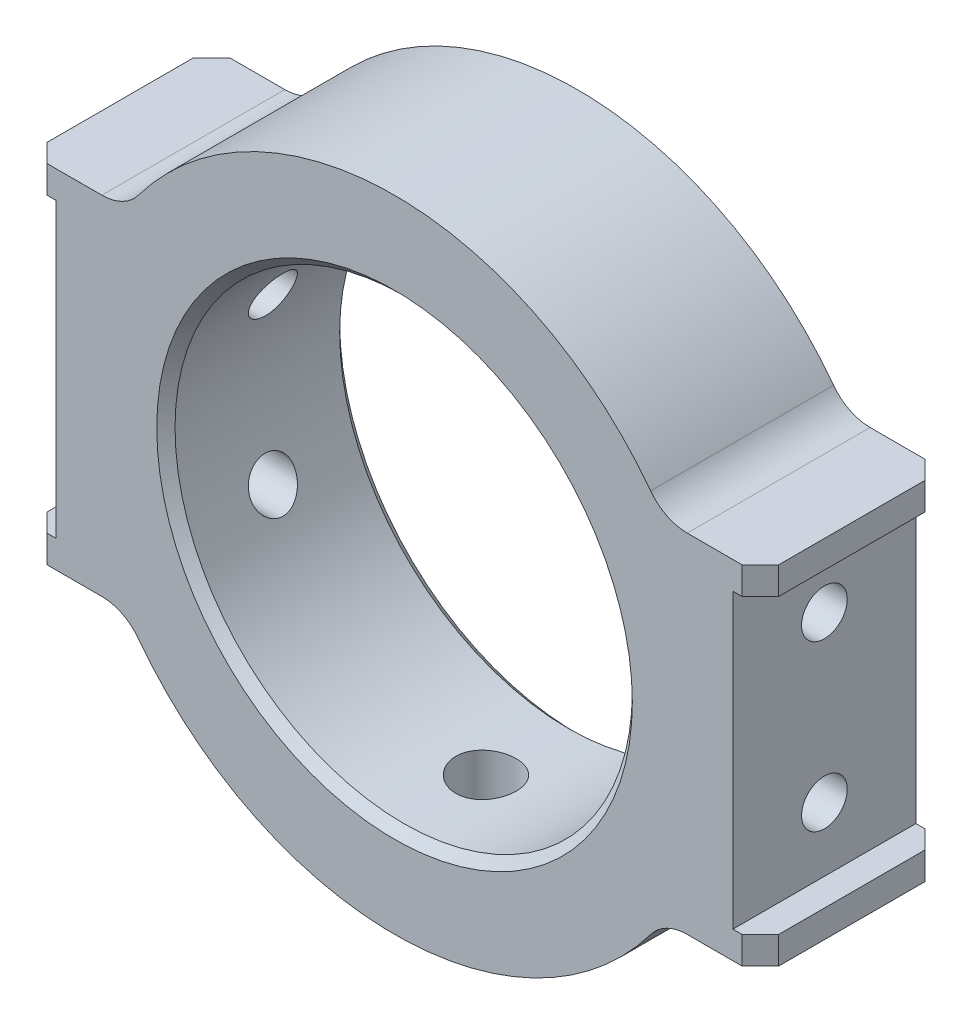
SolidWorks part; units mm, degrees
ref_plane "Front Plane" through (0, 0, 0) normal (0, 0, 1) x (1, 0, 0)
ref_plane "Top Plane" through (0, 0, 0) normal (0, 1, 0) x (1, 0, 0)
ref_plane "Right Plane" through (0, 0, 0) normal (1, 0, 0) x (0, 0, -1)
sketch "Sketch1" plane through (0, 0, 0) normal (0, 0, 1) x (1, 0, 0)
  circle A0 centre (0, 0) radius 17.5
  dimension "D1" = 35
extrude "Boss-Extrude1" add sketch "Sketch1" along normal blind 10
sketch "Sketch2" plane through (0, 0, 10) normal (0, 0, 1) x (1, 0, 0)
  line L1 (-20, -9.5) -> (20, -9.5)
  line L2 (-20, -9.5) -> (-20, 9.5)
  line L3 (-20, 9.5) -> (20, 9.5)
  line L4 (20, -9.5) -> (20, 9.5)
  line L5 (-20, -9.5) -> (20, 9.5) construction
  line L6 (-20, 9.5) -> (20, -9.5) construction
  point P0 (0, 0)
  dimension "D1" = 19
  dimension "D2" = 40
extrude "Boss-Extrude2" add sketch "Sketch2" against normal up to surface (10 mm away) up to face at (17.5, 0, 0)
chamfer "Chamfer1" distance 1 angle 45 4 edges at (20, 0, 0) (20, 0, 10) (-20, 0, 0) (-20, 0, 10)
sketch "Sketch3" plane through (0, 0, 10) normal (0, 0, 1) x (1, 0, 0)
  circle A0 centre (0, 0) radius 12.5
  dimension "D1" = 25
extrude "Cut-Extrude1" cut sketch "Sketch3" against normal through all
sketch "Sketch4" plane through (0, 0, 10) normal (0, 0, 1) x (1, 0, 0)
  line L0 (20, -9.5) -> (20, 9.5) construction
  line L1 (21.5, -8) -> (18.5, -8)
  line L2 (21.5, -8) -> (21.5, 8)
  line L3 (21.5, 8) -> (18.5, 8)
  line L4 (18.5, -8) -> (18.5, 8)
  line L5 (21.5, -8) -> (18.5, 8) construction
  line L6 (21.5, 8) -> (18.5, -8) construction
  line L7 (-20, 9.5) -> (-20, -9.5) construction
  line L8 (-21.5, -8) -> (-18.5, -8)
  line L9 (-21.5, -8) -> (-21.5, 8)
  line L10 (-21.5, 8) -> (-18.5, 8)
  line L11 (-18.5, -8) -> (-18.5, 8)
  line L12 (-21.5, -8) -> (-18.5, 8) construction
  line L13 (-21.5, 8) -> (-18.5, -8) construction
  point P0 (20, 0)
  point P7 (-20, 0)
  dimension "D1" = 16
  dimension "D2" = 1.5
extrude "Cut-Extrude2" cut sketch "Sketch4" against normal through all
ref_plane "Plane1" through (0, -20.3528, 0) normal (0, 1, 0) x (1, 0, 0)
hole_wizard "M4 Tapped Hole1" positions "Sketch6" profile "Sketch5" tap size "M4" standard "Gb"
sketch "Sketch6" plane through (0, -20.3528, 0) normal (0, 1, 0) x (1, 0, 0)
  line L0 (0, -10) -> (0, 0) construction
  line L1 (-14.6969, -10) -> (14.6969, -10) construction
  point P0 (0, -5)
sketch "Sketch5" plane through (0, -20.3528, 5) normal (1, 0, 0) x (0, 0, -1)
  line L0 (0, 0) -> (0, 11.0914)
  line L1 (0, 11.0914) -> (1.65, 10.1)
  line L2 (1.65, 10.1) -> (1.65, 0)
  line L5 (1.65, 0) -> (0, 0)
  line L10 (0, 11.0914) -> (-1.65, 10.1) construction
  line L11 (0, -6.35) -> (0, 107.95) construction
  dimension "螺纹孔钻头直径" = 3.3
  dimension "螺纹孔钻头深度" = 10.1
  dimension "导头角度" = 118
cosmetic thread "Hole thread 1" parameters "D1"=7.9622, "D2"=4
fillet "Fillet1" radius 2.5 4 edges at (14.6969, 9.5, 5) (-14.6969, 9.5, 5) (-14.6969, -9.5, 5) (14.6969, -9.5, 5)
hole_wizard "M3 Tapped Hole1" positions "Sketch8" profile "Sketch7" tap size "M3" standard "Gb"
sketch "Sketch8" plane through (18.5, 0, 0) normal (1, 0, 0) x (0, 0, -1)
  line L0 (-5, -8) -> (-5, 8) construction
  line L1 (0, -8) -> (-10, -8) construction
  line L2 (-1, 8) -> (-9, 8) construction
  line L4 (-5, 0) -> (-13.3246, 0) construction
  point P0 (-5, -4.5)
  point P2 (-5, 4.5)
  dimension "D1" = 9
sketch "Sketch7" plane through (18.5, -4.5, 5) normal (0, 1, 0) x (0, 0, -1)
  line L0 (0, 0) -> (0, 8.2511)
  line L1 (0, 8.2511) -> (1.25, 7.5)
  line L2 (1.25, 7.5) -> (1.25, 0)
  line L5 (1.25, 0) -> (0, 0)
  line L10 (0, 8.2511) -> (-1.25, 7.5) construction
  line L11 (0, -6.35) -> (0, 107.95) construction
  dimension "螺纹孔钻头直径" = 2.5
  dimension "螺纹孔钻头深度" = 7.5
  dimension "导头角度" = 118
cosmetic thread "Hole thread 2" parameters "D1"=6, "D2"=3
cosmetic thread "Hole thread 3" parameters "D1"=6, "D2"=3
mirror "Mirror1" about plane through (0, 0, 0) normal (1, 0, 0) of "M3 Tapped Hole1"
chamfer "Chamfer2" distance 0.5 angle 45 2 edges at (12.5, 0, 0) (12.5, 0, 10)
